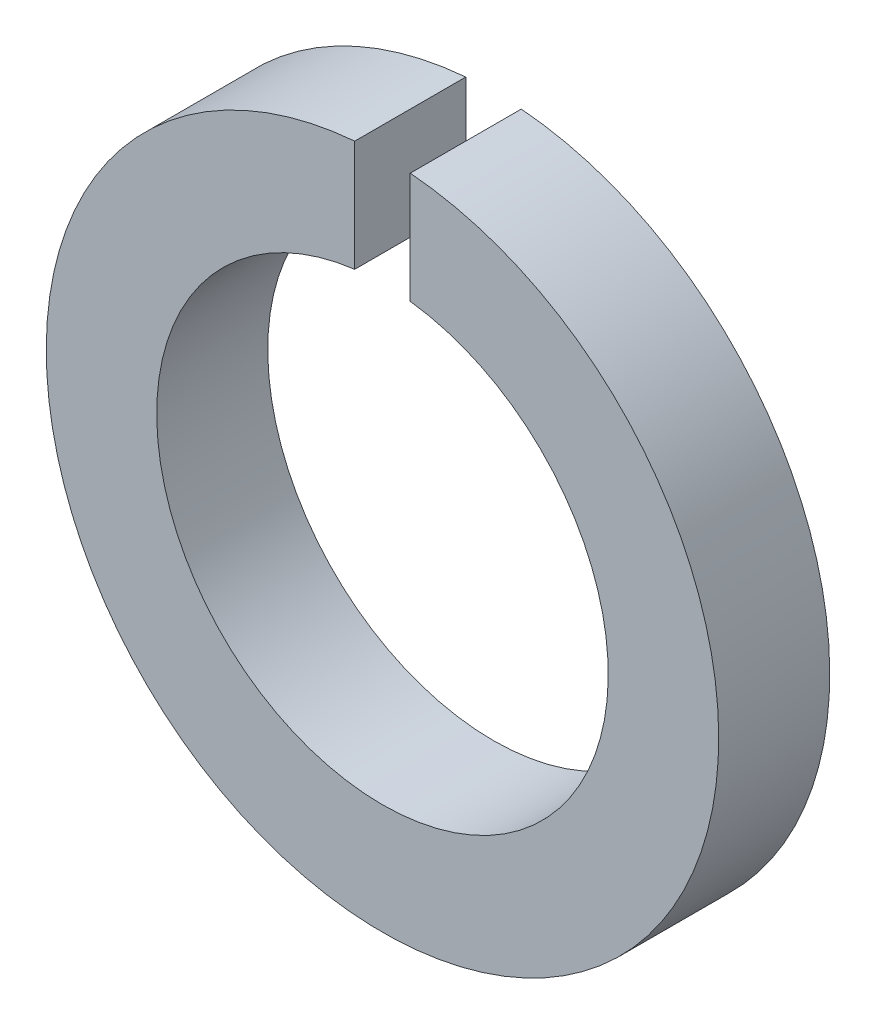
from build123d import *

# Parameters (mm, degrees)
EXTRUDE_1_DEPTH = 7.5


with BuildPart() as part:
    # Sketch 266 → 拉伸1 (new body)
    with BuildSketch(Plane.XY):
        with BuildLine():
            Line((-1.875, 22.634294665), (-1.875, 15.134294665))
            ThreePointArc((-1.875, 15.134294665), (0, -15.25), (1.875, 15.134294665))
            Line((1.875, 15.134294665), (1.875, 22.634294665))
            ThreePointArc((1.875, 22.634294665), (0, -22.711823352), (-1.875, 22.634294665))
        make_face()
    extrude(amount=EXTRUDE_1_DEPTH)


solid = part.part
